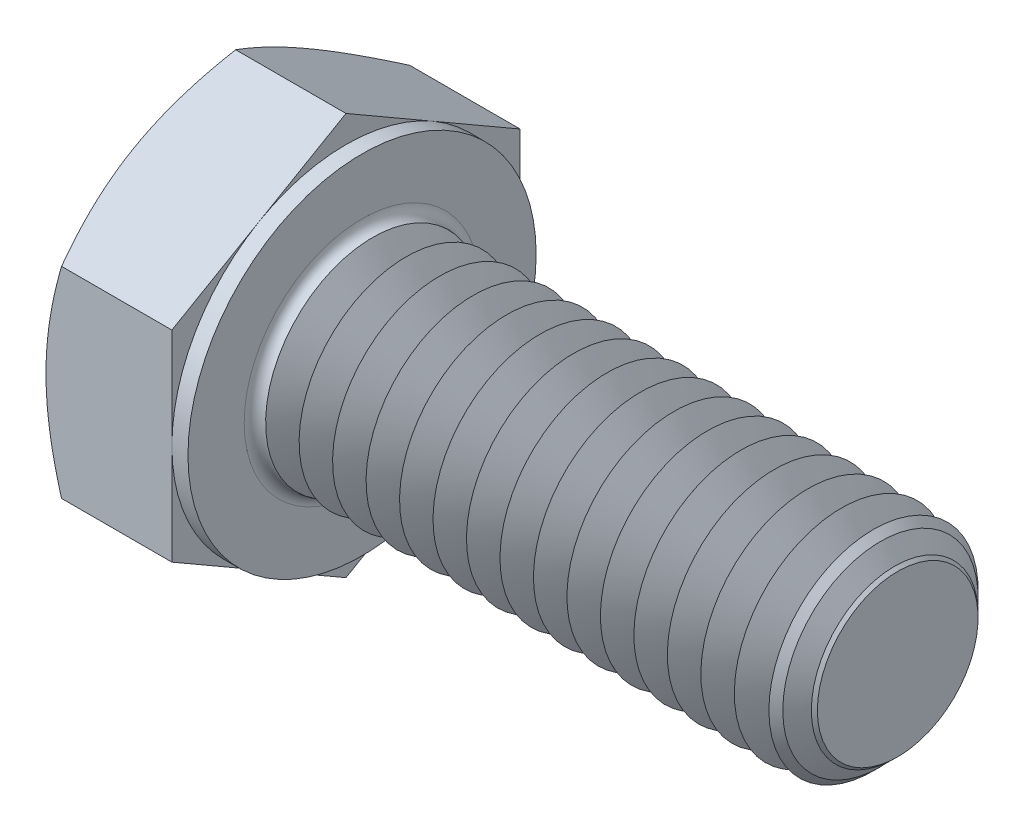
from build123d import *

# Parameters (mm, degrees)
EXTRUDE_374_DEPTH      = 5.3
SKETCH_4_W             = 0.6
SKETCH_4_H             = 11.005553499
CHAMFER_1917_SIZE      = 1
FILLET_1962_R          = 0.4
PATTERN_LINEAR_1_COUNT = 16
PATTERN_LINEAR_1_PITCH = 1.25


with BuildPart() as part:
    # 草图1 → Extrude 374 (new body)
    with BuildSketch(Plane(origin=(0, 0, 0), x_dir=(0, 0, -1), z_dir=(1, 0, 0))):
        Polygon((6.5, 3.75277675), (6.5, -3.75277675), (0, -7.505553499), (-6.5, -3.75277675), (-6.5, 3.75277675), (0, 7.505553499), align=None)
    extrude(amount=EXTRUDE_374_DEPTH)

    # 草图2 → 凸台-旋转1 (revolve)
    with BuildSketch(Plane.XY, mode=Mode.PRIVATE) as revolve_1_sk:
        Polygon((0, 0), (25.3, 0), (25.3, 2.9175), (25.3, 4), (0, 4), align=None)
    revolve(revolve_1_sk.sketch.rotate(Axis((0, 0, 0), (1, 0, 0)), 90), axis=Axis((0, 0, 0), (1, 0, 0)))

    # 草图3 → 切除-旋转1 (revolve, cut)
    with BuildSketch(Plane.XY):
        Polygon((0, 6.5), (3.46730793, 12.505553499), (3.46730793, 17.505553499), (-10, 17.505553499), (-10, 6.5), align=None)
    revolve(axis=Axis((0, 0, 0), (1, 0, 0)), mode=Mode.SUBTRACT)

    # 草图5 → 切除-旋转2 (revolve, cut)
    with BuildSketch(Plane.XY):
        Polygon((5.3, 6.5), (1.83269207, 12.505553499), (1.83269207, 17.505553499), (11.83269207, 17.505553499), (11.83269207, 6.5), align=None)
    revolve(axis=Axis((0, 0, 0), (1, 0, 0)), mode=Mode.SUBTRACT)

    # 草图4 → 切除-旋转3 (revolve, cut)
    with BuildSketch(Plane.XY, mode=Mode.PRIVATE) as cut_revolve_3_sk:
        with Locations((5, 12.00277675)):
            Rectangle(SKETCH_4_W, SKETCH_4_H)
    revolve(cut_revolve_3_sk.sketch.rotate(Axis((0, 0, 0), (1, 0, 0)), 270), axis=Axis((0, 0, 0), (1, 0, 0)), mode=Mode.SUBTRACT)

    # Chamfer 1917
    chamfer_1917_edges = [part.edges().sort_by_distance(p)[0] for p in [
        (25.3, 0, -4),
    ]]
    chamfer(chamfer_1917_edges, length=CHAMFER_1917_SIZE)

    # Fillet 1962
    fillet_1962_edges = [part.edges().sort_by_distance(p)[0] for p in [
        (5.3, 0, -4),
    ]]
    fillet(fillet_1962_edges, radius=FILLET_1962_R)

    # 草图6 → 切除-旋转4 (revolve, cut)
    with BuildSketch(Plane.XY):
        Polygon((6.324981666, -2.9175), (5.7, -4), (5.7, -5), (6.949963333, -5), (6.949963333, -4), align=None)
    cut_revolve_4 = revolve(axis=Axis((-3.175, 0, 0), (1, 0, 0)), mode=Mode.SUBTRACT)

    # 阵列(线性)1: 切除-旋转4 ×16
    with Locations(*[(i * PATTERN_LINEAR_1_PITCH, 0, 0) for i in range(1, PATTERN_LINEAR_1_COUNT)]):
        add(cut_revolve_4, mode=Mode.SUBTRACT)


solid = part.part
